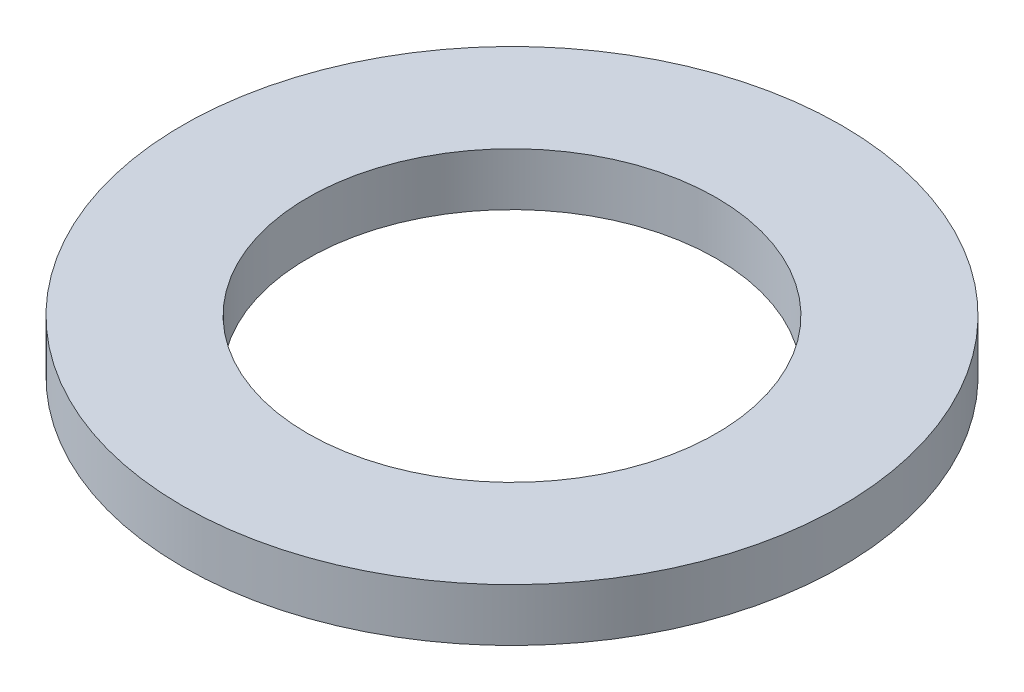
from build123d import *

# Parameters (mm, degrees)
SKETCH_1_R      = 25
SKETCH_1_R_2    = 15.5
EXTRUDE_1_DEPTH = 2


with BuildPart() as part:
    # 草图1 → 凸台-拉伸1 (new, symmetric)
    with BuildSketch(Plane(origin=(0, 0, 0), x_dir=(1, 0, 0), z_dir=(0, 1, 0))):
        with Locations(Location((0, 0, 0), (0, 0, 270))):
            Circle(SKETCH_1_R)
        with Locations(Location((0, 0, 0), (0, 0, 270))):
            Circle(SKETCH_1_R_2, mode=Mode.SUBTRACT)
    extrude(amount=EXTRUDE_1_DEPTH, both=True)


solid = part.part
